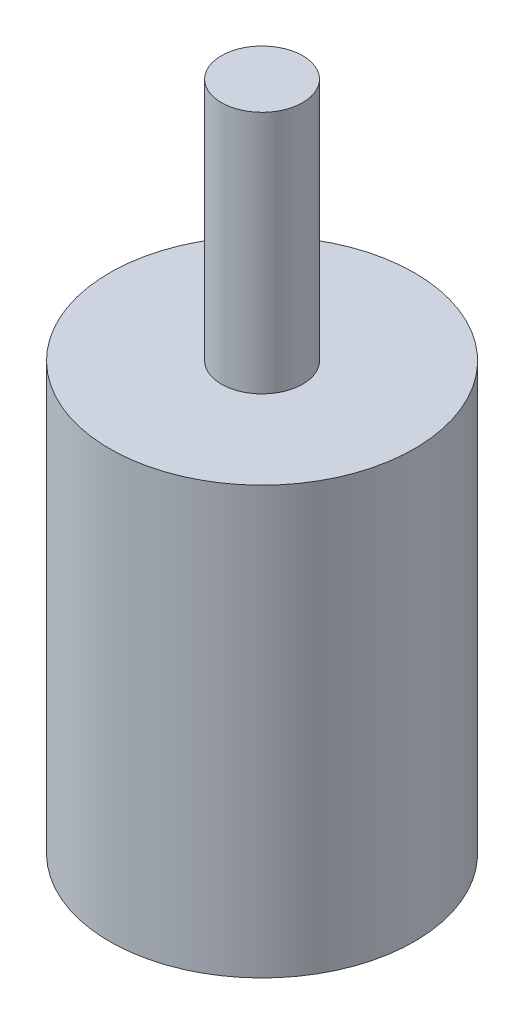
from build123d import *


with BuildPart() as part:
    # 草图1 → 旋转1 (revolve)
    with BuildSketch(Plane.XY, mode=Mode.PRIVATE) as revolve_1_sk:
        Polygon((0, 11.264150943), (2, 11.264150943), (2, -0.735849057), (7.5, -0.735849057), (7.5, -21.735849057), (0, -21.735849057), align=None)
    revolve(revolve_1_sk.sketch.rotate(Axis((0, 0, 0), (0, 1, 0)), 90), axis=Axis((0, 0, 0), (0, 1, 0)))


solid = part.part
